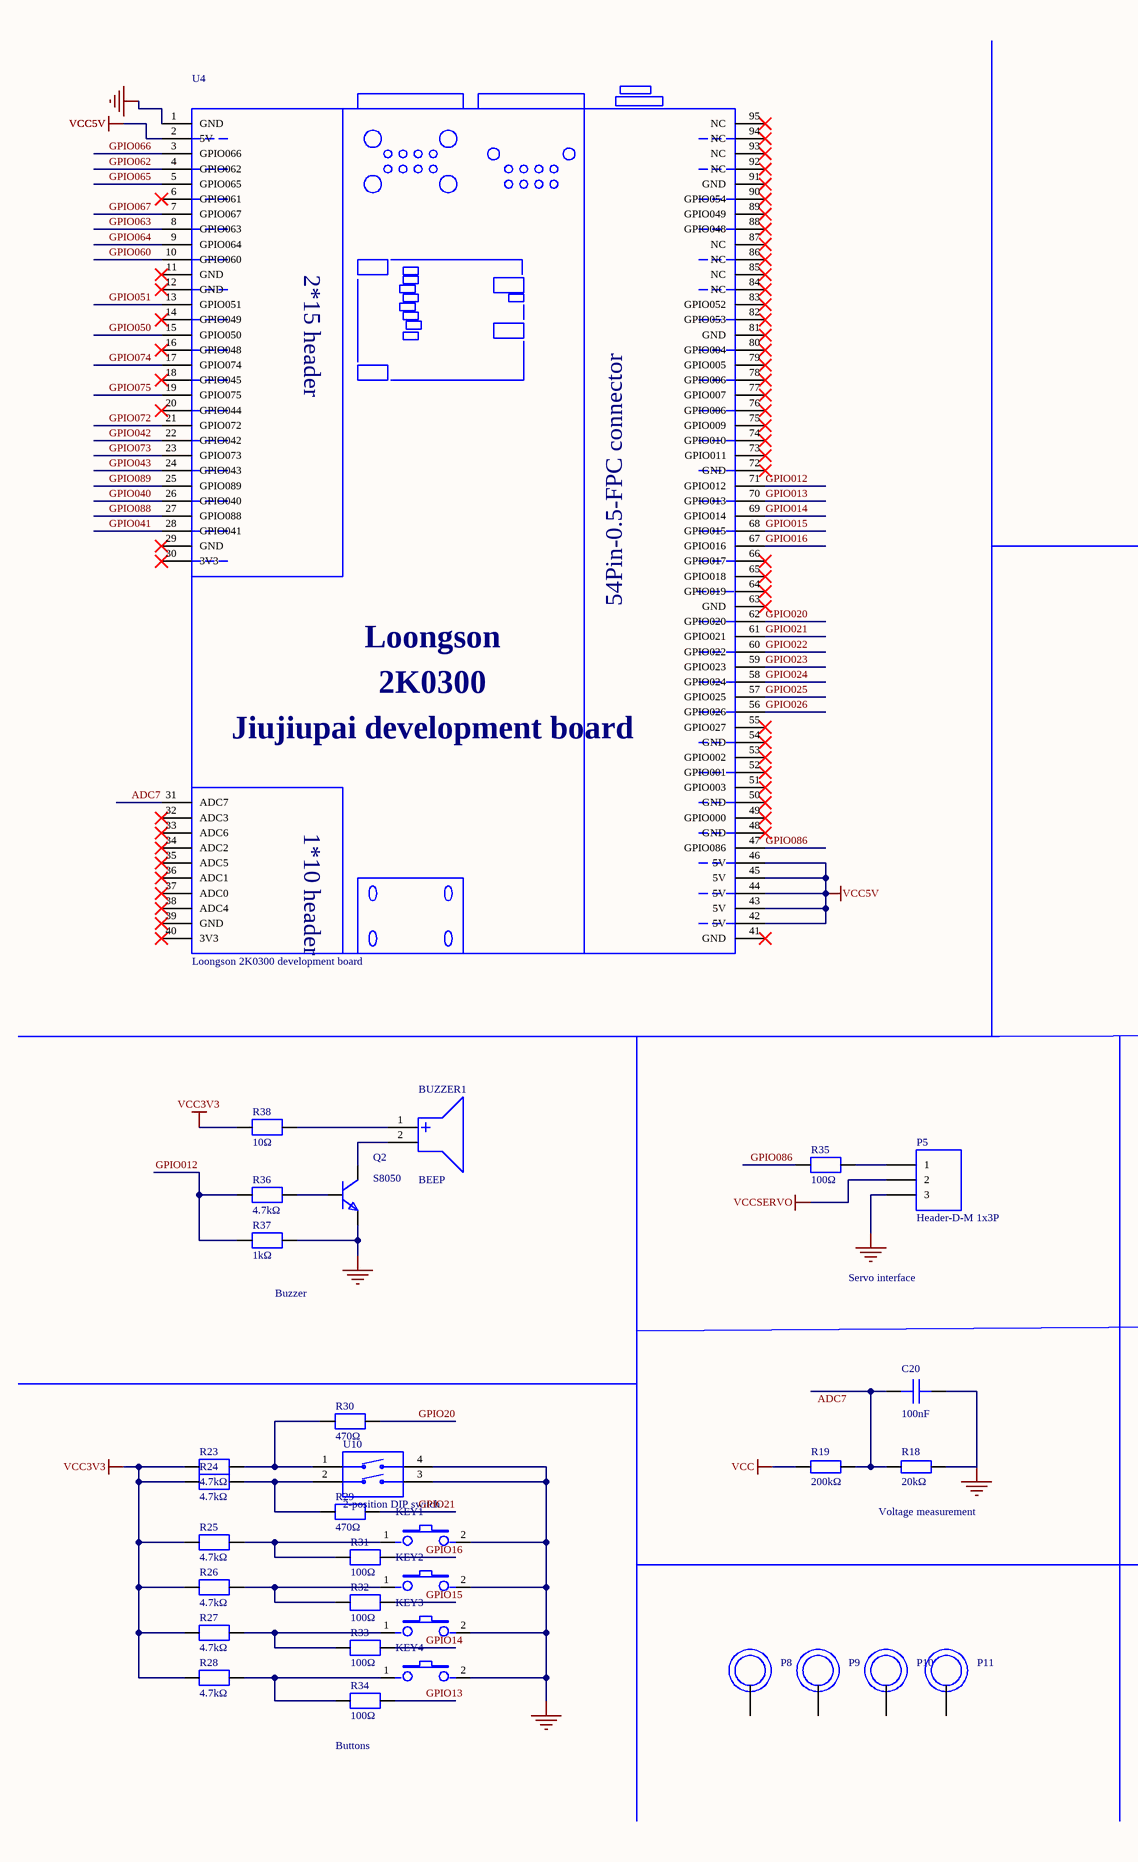
[diagram p0: MISC62349-3.schdoc, left]
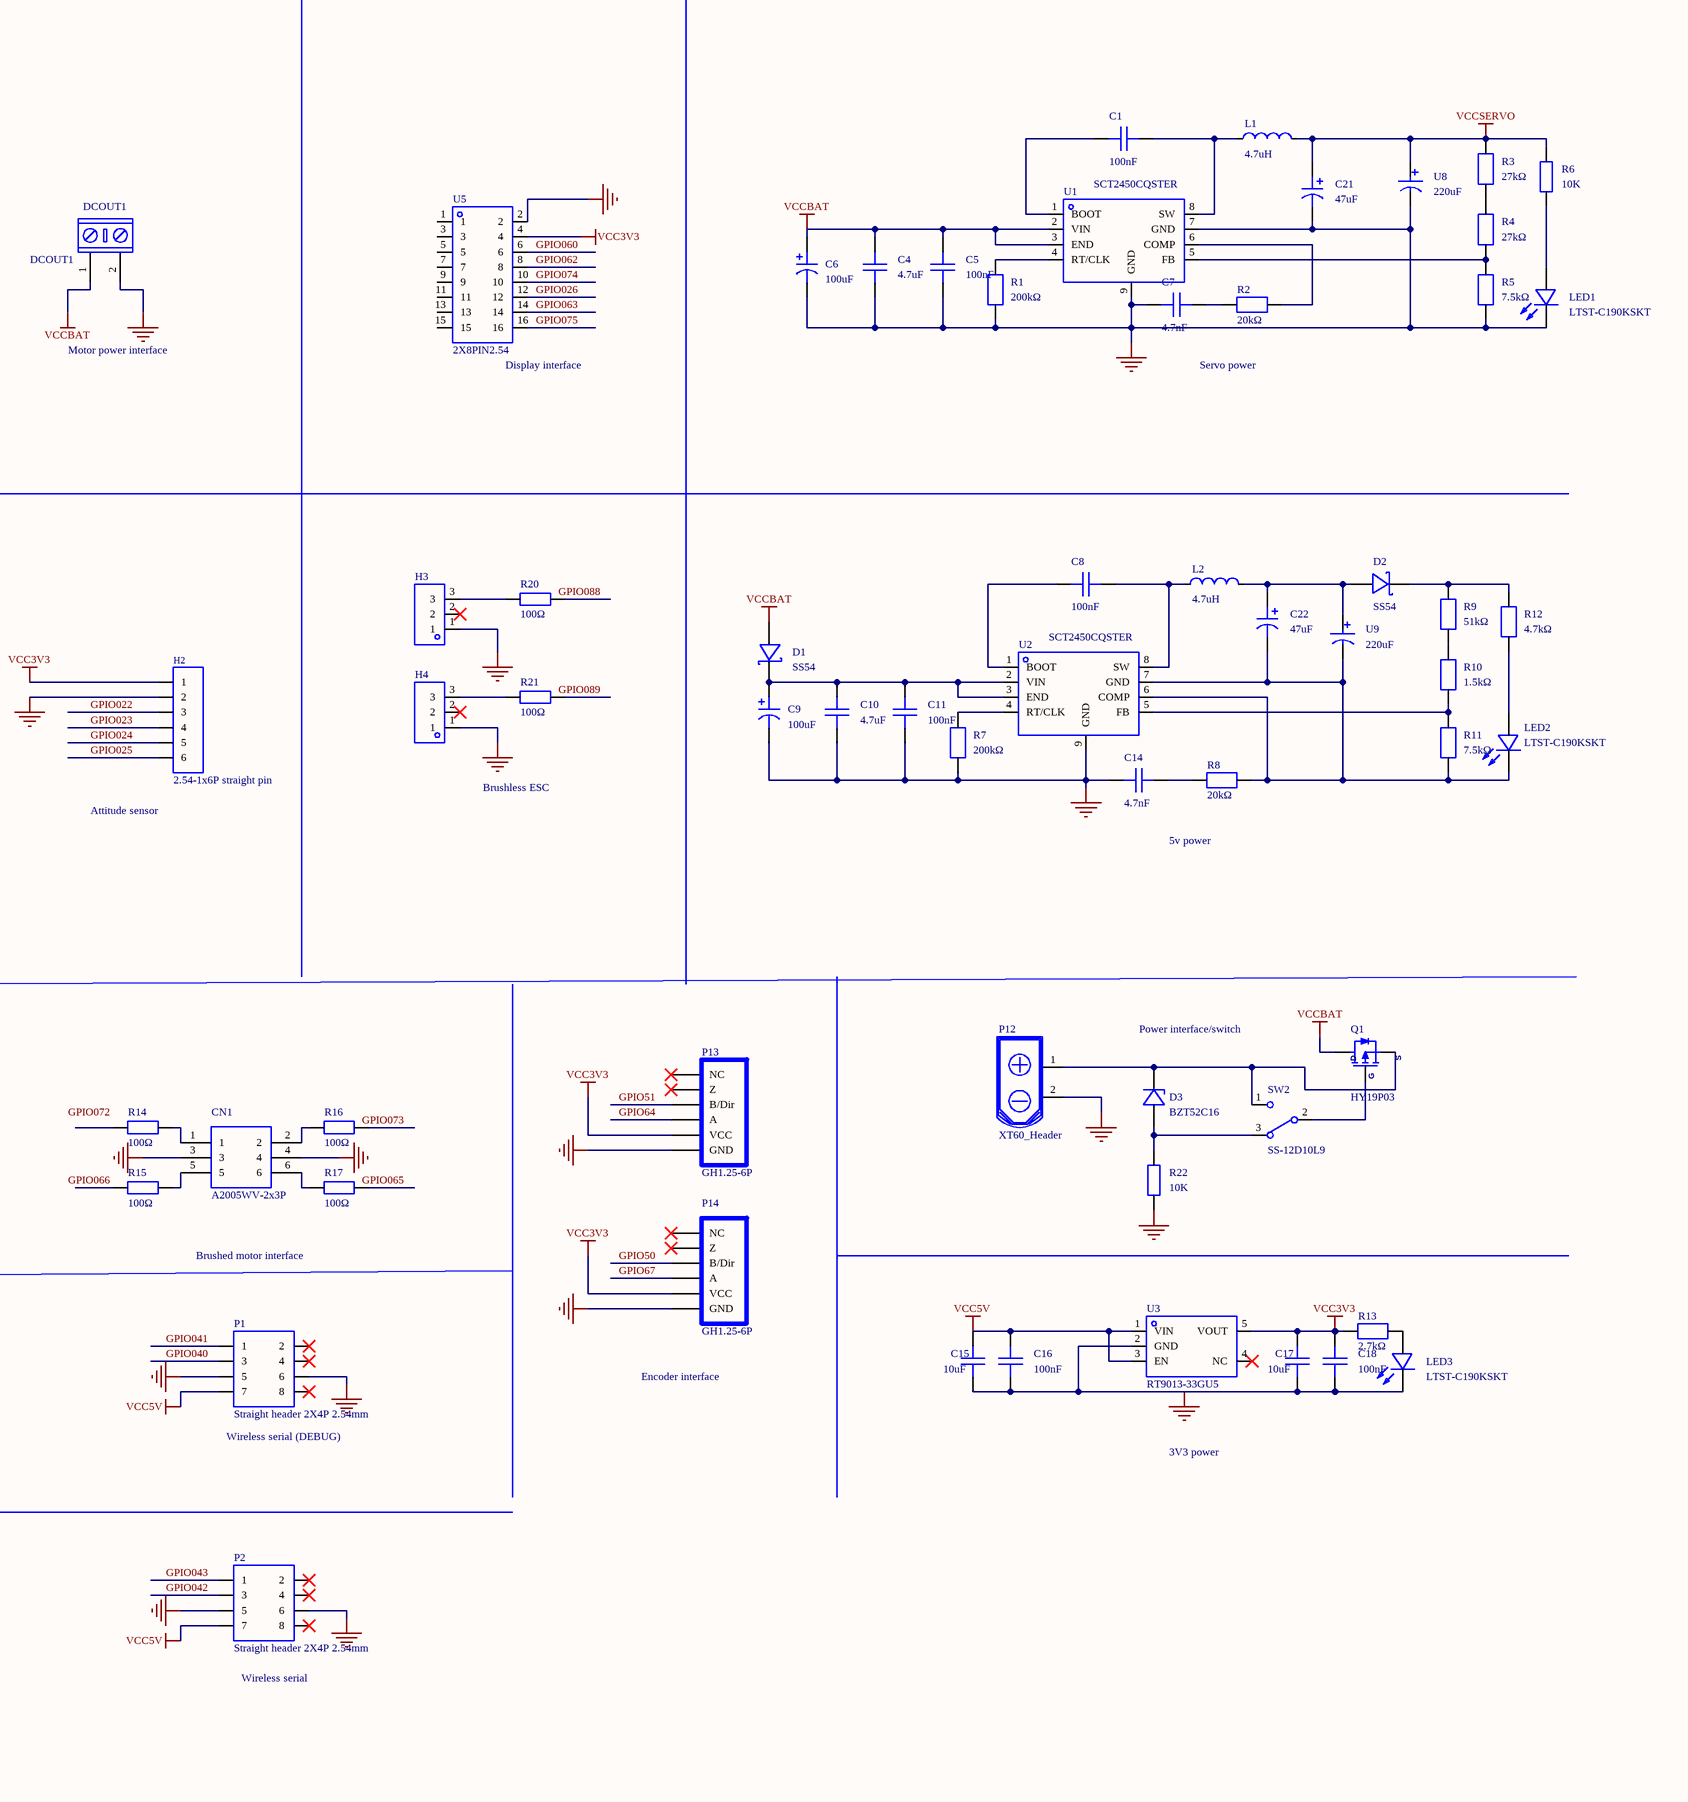
[diagram p1: MISC62349-3.schdoc, right]
# Altium project MISC62349-2.PrjPcb
1 sheet, 94 parts. Net scope: global (net labels, ports and power ports of the same name join across sheets).
Board file: MISC62349.pcbdoc

## Sheet MISC62349-3.schdoc
size 457 x 305 mm; Version: V1.0; @Project Name: MISC62349; @Page Count: 1; @Update Date: 2025-06-04; @Create Date: 2025-06-04; @Schematic Name: MISC62349; @Page No: 1; @Create Time: 18:07:27; @Update Time: 20:53:52; @Board Name: MISC62349

### Parts
BUZZER1  BEEP  [BUZ-TH_BD9-P50-D0.6-FD]
C1  100nF  [C0603]
C4  4.7uF  [C0402]
C5  100nF  [C0603]
C6  100uF  [CAP-SMD_L3.5-W2.8-R-RD]
C7  4.7nF  [C0603]
C8  100nF  [C0603]
C9  100uF  [CAP-SMD_L3.5-W2.8-R-RD]
C10  4.7uF  [C0402]
C11  100nF  [C0603]
C14  4.7nF  [C0603]
C15  10uF  [C0805]
C16  100nF  [C0603]
C17  10uF  [C0805]
C18  100nF  [C0603]
C20  100nF  [C0603]
C21  47uF  [CAP-SMD_BD6.3-L6.6-W6.6-LS7.3-FD]
C22  47uF  [CAP-SMD_BD6.3-L6.6-W6.6-LS7.3-FD]
CN1  A2005WV-2x3P  [HDR-TH_6P-P2.00-V-M-R2-C3-S2.00]
D1  SS54  [SMA_L4.4-W2.8-LS5.4-R-RD]
D2  SS54  [SMA_L4.4-W2.8-LS5.4-R-RD]
D3  BZT52C16  [SOD-123-L]
DCOUT1  DCOUT1  [KF/WJ/DG 301-2P-5.0MM]
H2  2.54-1x6P straight pin  [HDR-TH_6P-P2.54-V-M-1]
H3  (no value)  [HDR-TH_3P-P2.54-V-M]
H4  (no value)  [HDR-TH_3P-P2.54-V-M]
KEY1  Tact switch 3x6x2.5mm  [SW-SMD_L6.0-W3.6-LS8.0]  (value not drawn)
KEY2  Tact switch 3x6x2.5mm  [SW-SMD_L6.0-W3.6-LS8.0]  (value not drawn)
KEY3  Tact switch 3x6x2.5mm  [SW-SMD_L6.0-W3.6-LS8.0]  (value not drawn)
KEY4  Tact switch 3x6x2.5mm  [SW-SMD_L6.0-W3.6-LS8.0]  (value not drawn)
L1  4.7uH  [IND-SMD_L7.0-W6.6_VCMT063T]
L2  4.7uH  [IND-SMD_L7.0-W6.6_VCMT063T]
LED1  LTST-C190KSKT  [LED0603-RD]
LED2  LTST-C190KSKT  [LED0603-RD]
LED3  LTST-C190KSKT  [LED0603-RD]
P1  Straight header 2X4P 2.54mm  [HDR-TH_8P-P2.54-V-M-R2-C4-S2.54]
P2  Straight header 2X4P 2.54mm  [HDR-TH_8P-P2.54-V-M-R2-C4-S2.54]
P5  Header-D-M 1x3P  [HDR1X3-M]
P8  (no value)  [定位孔]
P9  (no value)  [定位孔]
P10  (no value)  [定位孔]
P11  (no value)  [定位孔]
P12  XT60_Header  [Wired T-Header ThroughHole]
P13  GH1.25-6P  [ECD-GH1.25-6P-SH]
P14  GH1.25-6P  [ECD-GH1.25-6P-SH]
Q1  HY19P03  [TO-252AA]
Q2  S8050  [SOT-23(SOT-23-3)]
R1  200kΩ  [R0603]
R2  20kΩ  [R0603]
R3  27kΩ  [R0603]
R4  27kΩ  [R0603]
R5  7.5kΩ  [R0603]
R6  10K  [R0603]
R7  200kΩ  [R0603]
R8  20kΩ  [R0603]
R9  51kΩ  [R0603]
R10  1.5kΩ  [R0603]
R11  7.5kΩ  [R0603]
R12  4.7kΩ  [R0603]
R13  2.7kΩ  [R0603]
R14  100Ω  [R0603]
R15  100Ω  [R0603]
R16  100Ω  [R0603]
R17  100Ω  [R0603]
R18  20kΩ  [R0603]
R19  200kΩ  [R0603]
R20  100Ω  [R0603]
R21  100Ω  [R0603]
R22  10K  [R0603]
R23  4.7kΩ  [R0603]
R24  4.7kΩ  [R0603]
R25  4.7kΩ  [R0603]
R26  4.7kΩ  [R0603]
R27  4.7kΩ  [R0603]
R28  4.7kΩ  [R0603]
R29  470Ω  [R0603]
R30  470Ω  [R0603]
R31  100Ω  [R0603]
R32  100Ω  [R0603]
R33  100Ω  [R0603]
R34  100Ω  [R0603]
R35  100Ω  [R0603]
R36  4.7kΩ  [R0603]
R37  1kΩ  [R0603]
R38  10Ω  [R0603]
SW2  SS-12D10L9  [MTS-10x]
U1  SCT2450CQSTER  [ESOP-8_L4.9-W3.9-P1.27-LS6.0-BL-EP]
U2  SCT2450CQSTER  [ESOP-8_L4.9-W3.9-P1.27-LS6.0-BL-EP]
U3  RT9013-33GU5  [SC-70-5_L2.0-W1.3-P0.65-LS2.1-BR]
U4  Loongson 2K0300 development board  [龙芯2K0300久久派开发板]
U5  2X8PIN2.54  [HDR-TH_16P-P2.54-V-M-R2-C8-S2.54]
U8  220uF  [CAP-SMD_BD6.3-L6.6-W6.6-LS7.2-FD]
U9  220uF  [CAP-SMD_BD6.3-L6.6-W6.6-LS7.2-FD]
U10  2-position DIP switch  [SW-TH_4P-L9.9-W6.8-P7.62-BL]

### Nets
GND: C4.1 C5.1 C6.2 C7.1 C9.2 C10.1 C11.1 C14.1 C15.1 C16.1 C17.1 C18.1 C20.2 C21.2 CN1.3 CN1.4 DCOUT1.2 H2.2 H3.1 H4.1 KEY1.2 KEY2.2 KEY3.2 KEY4.2 LED1.1(-) LED3.1(-) P1.5 P1.6 P2.5 P2.6 P5.3 P12.2(-) P13.1(GND) P14.1(GND) Q2.2(E) R1.1 R5.1 R7.1 R18.2 R22.1 R37.2 U1.7(GND) U1.9(GND) U2.9(GND) U3.2(GND) U4.1(GND) U5.2 U8.2 U10.3 U10.4
VCC: R19.1
VCC3V3: C17.2 C18.2 H2.1 P13.2(VCC) P14.2(VCC) R13.1 R23.1 R24.1 R25.1 R26.1 R27.1 R28.1 R38.1 U3.5(VOUT) U5.4
VCC5V: C15.2 C16.2 P1.7 P2.7 U3.1(VIN) U3.3(EN) U4.2(5V) U4.42(5V) U4.43(5V) U4.44(5V) U4.45(5V) U4.46(5V)
VCCBAT: C4.2 C5.2 C6.1 D1.1(A) DCOUT1.1 Q1.1(D) U1.2(VIN) U1.3(END)
VCCSERVO: C21.1 L1.2 P5.2 R3.2 R6.2 U8.1
ADC7: C20.1 R18.1 R19.2 U4.31(ADC7)
GPIO012: U4.71(GPIO012)
GPIO013: U4.70(GPIO013)
GPIO13: R34.2
GPIO014: U4.69(GPIO014)
GPIO14: R33.2
GPIO015: U4.68(GPIO015)
GPIO15: R32.2
GPIO016: U4.67(GPIO016)
GPIO16: R31.2
GPIO020: U4.62(GPIO020)
GPIO20: R30.2
GPIO021: U4.61(GPIO021)
GPIO21: R29.2
GPIO022: H2.3 U4.60(GPIO022)
GPIO023: H2.4 U4.59(GPIO023)
GPIO024: H2.5 U4.58(GPIO024)
GPIO025: H2.6 U4.57(GPIO025)
GPIO026: U4.56(GPIO026) U5.12
GPIO040: P1.3 U4.26(GPIO040)
GPIO041: P1.1 U4.28(GPIO041)
GPIO042: P2.3 U4.22(GPIO042)
GPIO043: P2.1 U4.24(GPIO043)
GPIO050: U4.15(GPIO050)
GPIO50: P14.4(B/Dir)
GPIO051: U4.13(GPIO051)
GPIO51: P13.4(B/Dir)
GPIO060: U4.10(GPIO060) U5.6
GPIO062: U4.4(GPIO062) U5.8
GPIO063: U4.8(GPIO063) U5.14
GPIO064: U4.9(GPIO064)
GPIO64: P13.3(A)
GPIO065: U4.5(GPIO065)
GPIO066: U4.3(GPIO066)
GPIO067: U4.7(GPIO067)
GPIO67: P14.3(A)
GPIO072: U4.21(GPIO072)
GPIO073: U4.23(GPIO073)
GPIO074: U4.17(GPIO074) U5.10
GPIO075: U4.19(GPIO075) U5.16
GPIO086: R35.1 U4.47(GPIO086)
GPIO088: U4.27(GPIO088)
GPIO089: U4.25(GPIO089)
NetBUZZER1_1: BUZZER1.1(+) R38.2
NetBUZZER1_2: BUZZER1.2(-) Q2.3(C)
NetC1_1: C1.1 U1.1(BOOT)
NetC1_2: C1.2 L1.1 U1.8(SW)
NetC7_2: C7.2 R2.2
NetC8_1: C8.1 U2.1(BOOT)
NetC8_2: C8.2 L2.1 U2.8(SW)
NetC9_1: C9.1 C10.2 C11.2 D1.2(K) U2.2(VIN) U2.3(END)
NetC14_2: C14.2 R8.2
NetC22_1: C22.1 D2.1(A) L2.2 U9.1
NetC22_2: C22.2 LED2.1(-) R8.1 R11.1 U2.6(COMP) U2.7(GND) U9.2
NetCN1_1: CN1.1 R14.2
NetCN1_2: CN1.2 R16.1
NetCN1_5: CN1.5 R15.2
NetCN1_6: CN1.6 R17.1
NetD2_2: D2.2(K) R9.2 R12.2
NetD3_A: D3.A R22.2 SW2.3
NetD3_K: D3.K P12.1(+) Q1.3(S) SW2.1
NetH3_3: H3.3 R20.1
NetH4_3: H4.3 R21.1
NetKEY1_1: KEY1.1 R25.2 R31.1
NetKEY2_1: KEY2.1 R26.2 R32.1
NetKEY3_1: KEY3.1 R27.2 R33.1
NetKEY4_1: KEY4.1 R28.2 R34.1
NetLED1_2: LED1.2(+) R6.1
NetLED2_2: LED2.2(+) R12.1
NetLED3_2: LED3.2(+) R13.2
NetP5_1: P5.1 R35.2
NetQ1_2: Q1.2(G) SW2.2
NetQ2_1: Q2.1(B) R36.2
NetR1_2: R1.2 U1.4(RT/CLK)
NetR2_1: R2.1 U1.6(COMP)
NetR3_1: R3.1 R4.2
NetR4_1: R4.1 R5.2 U1.5(FB)
NetR7_2: R7.2 U2.4(RT/CLK)
NetR9_1: R9.1 R10.2
NetR10_1: R10.1 R11.2 U2.5(FB)
NetR23_2: R23.2 R30.1 U10.1
NetR24_2: R24.2 R29.1 U10.2
NetR36_1: R36.1 R37.1

Not connected (* = marked no-connect by the designer): H3 2*; H4 2*; P1 2* 4* 8*; P2 2* 4* 8*; P8 1; P9 1; P10 1; P11 1; P13 5(Z)* 6(NC)*; P14 5(Z)* 6(NC)*; R14 1; R15 1; R16 2; R17 2; R20 2; R21 2; U3 4(NC)*; U4 6(GPIO061)* 11(GND)* 12(GND)* 14(GPIO049)* 16(GPIO048)* 18(GPIO045)* 20(GPIO044)* 29(GND)* 30(3V3)* 32(ADC3)* 33(ADC6)* 34(ADC2)* 35(ADC5)* 36(ADC1)* 37(ADC0)* 38(ADC4)* 39(GND)* 40(3V3)* 41(GND)* 48(GND)* 49(GPIO000)* 50(GND)* 51(GPIO003)* 52(GPIO001)* 53(GPIO002)* 54(GND)* 55(GPIO027)* 63(GND)* 64(GPIO019)* 65(GPIO018)* 66(GPIO017)* 72(GND)* 73(GPIO011)* 74(GPIO010)* 75(GPIO009)* 76(GPIO006)* 77(GPIO007)* 78(GPIO006)* 79(GPIO005)* 80(GPIO004)* 81(GND)* 82(GPIO053)* 83(GPIO052)* 84(NC)* 85(NC)* 86(NC)* 87(NC)* 88(GPIO048)* 89(GPIO049)* 90(GPIO054)* 91(GND)* 92(NC)* 93(NC)* 94(NC)* 95(NC)*; U5 1 3 5 7 9 11 13 15

### Notes on the sheet
- Motor power interface
- (near U5) Display interface
- Servo power
- (near H2) Attitude sensor
- Brushless ESC
- 5v power
- Power interface/switch
- (near R37) Buzzer
- Servo interface
- Brushed motor interface
- (near P1) Wireless serial (DEBUG)
- Encoder interface
- Voltage measurement
- 3V3 power
- (near R34) Buttons
- (near P2) Wireless serial
- Labels drawn without touching a wire or pin: GPIO012, GPIO065, GPIO066, GPIO072, GPIO073, GPIO088, GPIO089
- 2025-06-04
- Schematic
- Board
- Sheet
- P1
- Drawn
- Reviewed
- Revision
- Size
- A4
- page 1 Total 1
- EDA

### Library data of the parts
BUZZER1 = BEEP: ManufacturerPart: 5V,管脚间距8mm,外径10mm,高9.5mm; AddInBom: yes; ModelId: 638ddae033e2460c89b09f6fe40a11c2; ModelName: BUZ-TH_BD9.0-P5.00-D0.6-L-FD; ModelTransform: 354.33,354.13,433.07,90,0,0,0,0,-212.6; Device: BEEP; LCSC Part Name: 5V,管脚间距8mm,外径10mm,高9.5mm; SupplierPart: C9900017013; Supplier Footprint: BEEP; Supplier: LCSC; ConvertToPcb: yes; SymbolName: BEEP; FootprintName: BUZ-TH_BD9-P50-D0.6-FD
C1 C5 C8 C11 C16 C18 = 06031C104K4T2A: Capacitance:100nF;Tolerance:±10%;Rated voltage:100V;Temp coefficient:X7R;; Manufacturer: Kyocera AVX; AddInBom: yes; ModelId: ac125912035d415993ca9572d50418b1; ModelName: C0603_L1.6-W0.8-H0.8; ModelTransform: 62.992,31.496,0,0,0,0,0,0,0; Tolerance: ±10%; Voltage Rating: 100V; Temperature Coefficient: X7R; Symbol: 06031C104K4T2A; Device: 06031C104K4T2A; LCSC Part Name: 100nF ±10% 100V; SupplierPart: C1880996; ManufacturerPart: 06031C104K4T2A; Supplier Footprint: 0603; JLCPCB Part Class: Extended library; Supplier: LCSC; ConvertToPcb: yes; FootprintName: C0603; Value: 100nF
C4 C10 = 0402X475M160NT: Capacitance:4.7uF;Tolerance:±20%;Rated voltage:16V;Temp coefficient:X5R;; Manufacturer: FH(风华); AddInBom: yes; ModelId: 36a51122f27c49738f86b3bfa98863e0; ModelName: C0402_L1.0-W0.5-H0.5; ModelTransform: 39.37,19.685,0,0,0,0,0,0,0; Tolerance: ±20%; Voltage Rating: 16V; Temperature Coefficient: X5R; Symbol: 0402X475M160NT; Device: 0402X475M160NT; LCSC Part Name: 4.7uF ±20% 16V; SupplierPart: C2936654; ManufacturerPart: 0402X475M160NT; Supplier Footprint: 0402; JLCPCB Part Class: Extended library; Datasheet: https://atta.szlcsc.com/upload/public/pdf/source/20211229/0F554F04CCCC73F7B111AB47B2AF3160.pdf; Supplier: LCSC; ConvertToPcb: yes; FootprintName: C0402; Value: 4.7uF
C6 C9 = 8TPE100MAZB: Capacitance:100uF;Tolerance:±20%;Rated voltage:8V;Equivalent series resistance (ESR):35mΩ@100kHz;; Manufacturer: PANASONIC(松下); AddInBom: yes; ModelId: 0dfcda272f9b43668c6086d3a08712ba; ModelName: CASE-B_L3.5-W2.8-H1.9; ModelTransform: 145.669,110.236,0,180,0,0,0,0,0; Tolerance: ±20%; Voltage Rating: 8V; Symbol: 8TPE100MAZB; Device: 8TPE100MAZB; LCSC Part Name: 100uF ±20% 8V MSL=3拆包后请尽快使用; SupplierPart: C2158532; ManufacturerPart: 8TPE100MAZB; Supplier Footprint: 1411; JLCPCB Part Class: Extended library; Datasheet: https://atta.szlcsc.com/upload/public/pdf/source/20180730/C242097_33E927DF965764BEE6DB6E1D200BB8FE.pdf; Supplier: LCSC; ConvertToPcb: yes; FootprintName: CAP-SMD_L3.5-W2.8-R-RD; Value: 100uF; Current - Leakage: -; Ripple Current: -; Equivalent Series Resistance(ESR): 35mΩ@100kHz; Operating Temperature: -55℃~+105℃
C7 C14 = 0603CG472J500NT: Capacitance:4.7nF;Tolerance:±5%;Rated voltage:50V;Temp coefficient:C0G;; Manufacturer: FH(风华); AddInBom: yes; ModelId: ac125912035d415993ca9572d50418b1; ModelName: C0603_L1.6-W0.8-H0.8; ModelTransform: 62.992,31.496,0,0,0,0,0,0,0; Tolerance: ±5%; Voltage Rating: 50V; Temperature Coefficient: C0G; Symbol: 0603CG472J500NT; Device: 0603CG472J500NT; LCSC Part Name: 4.7nF ±5% 50V; SupplierPart: C20624280; ManufacturerPart: 0603CG472J500NT; Supplier Footprint: 0603; JLCPCB Part Class: Extended library; Datasheet: https://atta.szlcsc.com/upload/public/pdf/source/20231013/50987BFA113EBC42343E989A0A057269.pdf; Supplier: LCSC; ConvertToPcb: yes; FootprintName: C0603; Value: 4.7nF
C15 C17 = C0805X106K8RACAUTO: Capacitance:10uF;Tolerance:±10%;Rated voltage:10V;Temp coefficient:X7R;; Manufacturer: KEMET(基美); AddInBom: yes; ModelId: 1ba041120af144c991958decab20d241; ModelName: C0805_L2.0-W1.3-H1.3; ModelTransform: 78.74,51.181,0,0,0,0,0,0.0005,0; Tolerance: ±10%; Voltage Rating: 10V; Temperature Coefficient: X7R; Symbol: C0805X106K8RACAUTO; Device: C0805X106K8RACAUTO; LCSC Part Name: 10uF ±10% 10V; SupplierPart: C2167871; ManufacturerPart: C0805X106K8RACAUTO; Supplier Footprint: 0805; JLCPCB Part Class: Extended library; Datasheet: https://atta.szlcsc.com/upload/public/pdf/source/20210401/7F57E742531715B36FE1E9CC2258952B.pdf; Supplier: LCSC; ConvertToPcb: yes; FootprintName: C0805; Value: 10uF
C20 = CAP_0603: ConvertToPcb: yes; SymbolName: CapAcitance; ModelId: ac125912035d415993ca9572d50418b1; ModelName: C0603_L1.6-W0.8-H0.8; ModelTransform: 62.992,31.496,0,0,0,0,0,0,0; Device: CAP_0603; AddInBom: yes; Supplier Footprint: 0603; FootprintName: C0603; Value: 100nF
C21 C22 = SPT1CM470E05TRVZC: Capacitance:47uF;Tolerance:±20%;Rated voltage:16V;Type:Polymer;; Manufacturer: Yunxing(云星); AddInBom: yes; ModelId: 697a8c63e3274188b68c96045bc3ea1c; ModelTransform: 287.401,259.842,0,180,0,0,0.001,0.001,0; Tolerance: ±20%; Voltage Rated: 16V; Lifetime @ Temp: 2000hrs@105℃; Symbol: SPT1CM470E05TRVZC; Device: SPT1CM470E05TRVZC; LCSC Part Name: 47uF ±20% 16V; SupplierPart: C41410186; ManufacturerPart: SPT1CM470E05TRVZC; Supplier Footprint: SMD,D6.3xL5mm; Datasheet: https://atta.szlcsc.com/upload/public/pdf/source/20240919/E10B786B053F2EF740092A8DAB1988C9.pdf; Supplier: LCSC; ConvertToPcb: yes; FootprintName: CAP-SMD_BD6.3-L6.6-W6.6-LS7.3-FD; ModelName: CAP-SMD_BD6.3-L6.6-W6.6-LS7.3-FD; Value: 47uF; Type: Polymer; Diameter: 6.3mm; Height - Seated (Max): 5mm; Operating Temperature: -55℃~+105℃
CN1 = A2005WV-2x3P: 间距:2mm;总PIN位数:6;排数:2;插针结构:2x3P;行距:2mm;安装类型:直插;圆针/方针:方针;额定电流:-;额定电压:-;配合针长度:4mm;塑高:-;端接针长度:2.8mm;触头材质:黄铜;触头镀层:金;工作温度范围:-40℃~+105℃;颜色:黑色;; Manufacturer: CJT(长江连接器); AddInBom: yes; ModelId: 7bb0589f04a2434cbd3f756f04868c86; ModelName: HDR-TH_6P-P2.00-M-LI-2X3P; ModelTransform: 236.22,157.48,0,0,0,0,0,0,-118.11; Pitch: 2mm; Pin Structure: 2x3P; Circluar Pins/Square Pins: Square pin; Device: A2005WV-2x3P; Symbol: A2005WV-2X3P; LCSC Part Name: 2mm 2x3P 直插 方针 镀金; SupplierPart: C225288; ManufacturerPart: A2005WV-2x3P; Supplier Footprint: 插件,P=2mm; JLCPCB Part Class: Extended Part; Datasheet: https://atta.szlcsc.com/upload/public/pdf/source/20180509/C225288_5A34F913C29FC1A6DA0E0F7E9D3856BA.pdf; Supplier: LCSC; ConvertToPcb: yes; FootprintName: HDR-TH_6P-P2.00-V-M-R2-C3-S2.00; Number of Pins: 6; Number of Rows: 2; Row Spacing: 2mm; Mounting Type: Through-hole; Current Rating (Max): -; Voltage Rating (Max): -; Length of Mating Pin: 4mm; Insulation Height: -; Length of End Connection Pin: 2.8mm; Contact Material: Brass; Contact Plating: Gold; Operating Temperature Range: -40℃~+105℃; Color: Black
D1 D2 = SS54_C22452: Diode configuration:Single;Forward voltage drop (Vf):550mV@5A;DC reverse voltage (Vr):40V;Rectified current:5A;; Manufacturer: MDD(辰达半导体); AddInBom: yes; ModelId: 228de99b63224bd3982b21290755dd84; ModelTransform: 204.724,110.236,0,0,0,0,0,0,0; Diode Configuration: Single; Reverse Voltage (Vr): 40V; Rectified Current: 5A; Reverse Leakage Current (Ir): 1mA@40V; Symbol: SS54_C22452; Device: SS54_C22452; LCSC Part Name: 电压:40V 电流:5A; SupplierPart: C22452; ManufacturerPart: SS54; Supplier Footprint: SMA(DO-214AC); JLCPCB Part Class: Basic library; Datasheet: https://atta.szlcsc.com/upload/public/pdf/source/20240710/73DFBB65C1883B895E62D589679033DF.pdf; Supplier: LCSC; ConvertToPcb: yes; FootprintName: SMA_L4.4-W2.8-LS5.4-R-RD; ModelName: SMA_L4.4-W2.8-LS5.4-R-RD; Forward Voltage (Vf@If): 550mV@5A
D3 = BZT52C16: Origin Footprint 2: DIODE-0.7; Origin Footprint 3: DIODE-0.4; Origin Footprint 4: SOD-87[LL-41]; Origin Footprint 5: CD4521-1808; Origin Footprint 6: SOD-80[LL-34]; Origin Footprint 7: SOD-123-FL; Origin Footprint 8: SOD-123-M; Origin Footprint 9: SOD-323; Origin Footprint 10: SOD-523-L; Origin Footprint 11: SOD-523-M; AddInBom: yes; SymbolName: Diode Zen; Device: BZT52C16; Published: 8-Jun-2000; Revision: July-2002: Re-released for DXP Platform.; Price(RMB): 0.000; ConvertToPcb: yes; FootprintName: SOD-123-L; Publisher: Altium Limited
DCOUT1 = DCOUT1: AddInBom: yes; Device: DCOUT1; ConvertToPcb: yes; SymbolName: DCOUT1; FootprintName: KF/WJ/DG 301-2P-5.0MM
H2 = 2.54-1x6P直针: 间距:2.54mm;总PIN位数:6;排数:1;插针结构:1x6P;行距:-;安装类型:直插;圆针/方针:方针;额定电流:3A;额定电压:-;配合针长度:-;塑高:-;触头材质:黄铜;触头镀层:-;工作温度范围:-40℃~+105℃;颜色:黑色;; Manufacturer: BOOMELE(博穆精密); Symbol: Header-Male-2.54_1x6; AddInBom: yes; ModelId: 60739dffc9b04830a286435b0fefbd4a; ModelName: HDR2.54-M-LI-1X6P; ModelTransform: 600,100,0,0,0,0,0,0,-118.1; Pitch: 2.54mm; Pin Structure: 1x6P; Circluar Pins/Square Pins: Square pin; Current Rating (Max): 3A; Device: 2.54-1x6P straight pin; Supplier: LCSC; Manufacturer Part: 2.54-1x6P直针; Supplier Part: C37208; JLCPCB Part Class: Extended Part; LCSC Part Name: 2.54mm 1x6P 直插 方针; Supplier Footprint: 直插,P=2.54mm; Datasheet: https://atta.szlcsc.com/upload/public/pdf/source/20151109/1457707558014.pdf; ConvertToPcb: yes; FootprintName: HDR-TH_6P-P2.54-V-M-1; Number of Pins: 6; Number of Rows: 1; Row Spacing: -; Mounting Type: Through-hole; Voltage Rating (Max): -; Length of Mating Pin: -; Insulation Height: -; Contact Material: Brass; Contact Plating: -; Operating Temperature Range: -40℃~+105℃; Color: Black
H3 H4 = HDR-M_2.54_1x3P: Symbol: PZ254V-11-03P_C2937625; ConvertToPcb: yes; ModelId: bb473b6d38ff42a99216a4fcdbdcc4cb; ModelName: HDR-TH_3P-P2.54-M-LI-1X3P; ModelTransform: 299.9994,100,0,0,0,0,0,0,-118.11; Device: HDR-M_2.54_1x3P; AddInBom: yes; SupplierPart: C2937625; Supplier Footprint: 插件; FootprintName: HDR-TH_3P-P2.54-V-M
KEY1-KEY4 = 轻触按键 3x6x2.5mm: AddInBom: yes; ModelId: 5cda64a5897044e48badc24f5aa7d420; ModelName: SW-SMD_L6.0-W3.6-H2.5-LS8.0; ModelTransform: 314.96,141.732,0,0,0,0,0,0,0; Symbol: 3x6x2.5mm; Device: Tact switch 3x6x2.5mm; LCSC Part Name: 3x6x2.5 红头 耐高温; SupplierPart: C5382; ManufacturerPart: 轻触按键 3x6x2.5mm; Supplier Footprint: SMD; JLCPCB Part Class: Extended library; Supplier: LCSC; ConvertToPcb: yes; FootprintName: SW-SMD_L6.0-W3.6-LS8.0
L1 L2 = ZEMS0603-4R7M: Inductance:4.7uH;Tolerance:±20%;Rated current:6A;Saturation current (Isat):9A;Type:Molded inductor;; Manufacturer: ZE(增益); AddInBom: yes; ModelId: f4285975b224408e9720a50707b42a76; ModelTransform: 275.59,260.2357,0,0,0,0,0,0,0; Tolerance: ±20%; Current Rating: 6A; Current - Saturation(Isat): 9A; DC Resistance(DCR): 40mΩ; Symbol: ZEMS0603-4R7M; Device: ZEMS0603-4R7M; LCSC Part Name: ZEMS0603-4R7M; SupplierPart: C41415578; ManufacturerPart: ZEMS0603-4R7M; Supplier Footprint: SMD,7x6.6mm; Datasheet: https://atta.szlcsc.com/upload/public/pdf/source/20241008/E174FBE73995C1DD66BAC4D7D2F842CD.pdf; Supplier: LCSC; ConvertToPcb: yes; FootprintName: IND-SMD_L7.0-W6.6_VCMT063T; ModelName: IND-SMD_L7.0-W6.6_VCMT063T; Value: 4.7uH; Type: Molded inductor
LED1-LED3 = LTST-C190KSKT: 发光颜色:黄色;正向电压(VF):2.1V;功率:75mW;正向电流:20mA;主波长:584.5nm~597nm;二极管配置:-;透镜颜色:无色透明透镜;色温:-;发光强度:104mcd;发光角度:130°;载带方式:-;工作温度:-30℃~+85℃;; Manufacturer: LITEON(光宝); AddInBom: yes; ModelId: 1f0d29a91be547639d425604e9b96ebb; ModelTransform: 63.7794,32.283,0,0,0,0,0,0,0; Emitted Color: Yellow; Forward Voltage (VF): 2.1V; Power Dissipation: 75mW; Forward Current: 20mA; Peak Wavelength: 588nm; Lens Color: Clear lens; Luminous Intensity: 104mcd; Viewing Angle: 130°; Symbol: LTST-C190KSKT; Device: LTST-C190KSKT; LCSC Part Name: 黄灯; SupplierPart: C125095; ManufacturerPart: LTST-C190KSKT; Supplier Footprint: 0603; JLCPCB Part Class: Extended library; Datasheet: https://atta.szlcsc.com/upload/public/pdf/source/20180129/C125095_15171881843821315881.pdf; Supplier: LCSC; ConvertToPcb: yes; FootprintName: LED0603-RD; ModelName: LED0603-RD; Dominant Wavelength: 584.5nm~597nm; Diode Configuration: -; Color Temperature: -; Mounting Sytle: -; Operating Temperature: -30℃~+85℃
P1 P2 = 直排针2X4P 2.54mm: Rows:-;Round/square pin:-;Rated current:-;Rated voltage:-;Mating pin length:-;Plastic height:-;Contact material:-;; Manufacturer: BOOMELE(博穆精密); Symbol: Header-Male-2.54_2x4; AddInBom: yes; ModelId: 9655140a9899454ea9d6a6732d55fb0e; ModelName: HDR-TH_8P-P2.54-M-LI-2X4P; ModelTransform: 400,200,0,0,0,0,0,0,-118.1; Device: Straight header 2X4P 2.54mm; LCSC Part Name: 排针 2*4P 2.54mm; SupplierPart: C58363; ManufacturerPart: 直排针2X4P 2.54mm; Supplier Footprint: 插件,P=2.54mm; JLCPCB Part Class: Extended Part; Datasheet: https://atta.szlcsc.com/upload/public/pdf/source/20151026/1457707506726.pdf; Supplier: LCSC; ConvertToPcb: yes; FootprintName: HDR-TH_8P-P2.54-V-M-R2-C4-S2.54; Number of Rows: -; Circluar Pins/Square Pins: -; Current Rating (Max): -; Voltage Rating (Max): -; Length of Mating Pin: -; Insulation Height: -; Contact Material: -
P5 = Header-D-M 1x3P: 1x3pin, through-hole, pin header; AddInBom: yes; Device: Header-D-M 1x3P; Revision: V1.0; Value: Header-D-M 1x3P; Footprint Name: HDR1X3-M; ConvertToPcb: yes; SymbolName: Header-D-M 1x3P; FootprintName: HDR1X3-M
P8-P11 = 定位孔: Device: Locating hole; AddInBom: yes; ModelId: c0272a1083aa488a8080554edf29f67b; ModelName: SMD_SMTSO3060CTJ; ModelTransform: 218.897,218.387,0,0,0,0,-0.155,-0.01,-59.055; _: 3; ConvertToPcb: yes; SymbolName: Locating hole; FootprintName: Locating hole
P12 = XT60_Header: AddInBom: yes; Device: XT60_Header; Footprint Name: XT60UF; ConvertToPcb: yes; SymbolName: XT60_Header; FootprintName: Wired T-Header ThroughHole; Description: XT60_Header
P13 P14 = GH1.25-6P: COMPANY_A 1024-line encoder GH1.25-6P, board side; AddInBom: yes; SymbolName: GH1.25-6P-new encoder board side; Device: GH1.25-6P; Revision: V1.0; Value: GH1.25-6P; Footprint Name: ECD-GH1.25-6P-SV; ConvertToPcb: yes; FootprintName: ECD-GH1.25-6P-SH
Q1 = HY19P03: AddInBom: yes; Device: HY19P03; ConvertToPcb: yes; SymbolName: HY19P03; FootprintName: TO-252AA
Q2 = S8050: Manufacturer: CJ; AddInBom: yes; Device: S8050; ConvertToPcb: yes; SymbolName: S8050; Supplier: LCSC; ManufacturerPart: S8050; image: C2146.jpg; SupplierPart: C2146; JLCPCB Part Class: Basic; FootprintName: SOT-23(SOT-23-3)
R1 R7 = AF0805FR-07200KL: Resistor type:Thick film resistor;Resistance:200kΩ;Tolerance:±1%;Power:125mW;Temp coefficient:±100ppm/℃;; Manufacturer: YAGEO(国巨); AddInBom: yes; ModelId: 37a81e68749a4138bd2dfa6897b24b85; ModelName: R0805_L2.0-W1.3-H0.6; ModelTransform: 78.74,51.181,0,0,0,0,0,-0.0005,0; Tolerance: ±1%; Power(Watts): 125mW; Symbol: AF0805FR-07200KL; Device: AF0805FR-07200KL; LCSC Part Name: 厚膜电阻 200kΩ ±1% 125mW; SupplierPart: C3957483; ManufacturerPart: AF0805FR-07200KL; Supplier Footprint: 0805; JLCPCB Part Class: Extended library; Datasheet: https://atta.szlcsc.com/upload/public/pdf/source/20240124/9D5CBAA83CB4685F032349418AF2E20F.pdf; Supplier: LCSC; ConvertToPcb: yes; FootprintName: R0603; Type: Thick film resistor; Value: 200kΩ; Temperature Coefficient: ±100ppm/℃; Operating Temperature: -55℃~+155℃
R2 R8 = MMA02040D2002FB300: Resistor type:Thin film resistor;Resistance:20kΩ;Tolerance:±1%;Power:400mW;Working voltage:200V;Temp coefficient:±25ppm/℃;; Manufacturer: VISHAY(威世); AddInBom: yes; ModelId: bdd6039e5cb54d129162151e55f23c33; ModelName: R0204; ModelTransform: 137.795,55.09383,0,0,0,0,0,0,0; Tolerance: ±1%; Power(Watts): 400mW; Voltage-Supply(Max): 200V; Symbol: MMA02040D2002FB300; Device: MMA02040D2002FB300; LCSC Part Name: 薄膜电阻 20kΩ ±1% 400mW; SupplierPart: C2139897; ManufacturerPart: MMA02040D2002FB300; Supplier Footprint: 0204; JLCPCB Part Class: Extended library; Datasheet: https://atta.szlcsc.com/upload/public/pdf/source/20210505/324368DA0CE91162B72B5E4004EB06CA.pdf; Supplier: LCSC; ConvertToPcb: yes; FootprintName: R0603; Type: Thin film resistor; Value: 20kΩ; Temperature Coefficient: ±25ppm/℃; Operating Temperature: -55℃~+155℃
R3 R4 = RT0805BRE0727KL: Resistor type:Thin film resistor;Resistance:27kΩ;Tolerance:±0.1%;Power:125mW;Temp coefficient:±50ppm/℃;; Manufacturer: YAGEO(国巨); AddInBom: yes; ModelId: 37a81e68749a4138bd2dfa6897b24b85; ModelName: R0805_L2.0-W1.3-H0.6; ModelTransform: 78.74,51.181,0,0,0,0,0,-0.0005,0; Tolerance: ±0.1%; Power(Watts): 125mW; Symbol: RT0805BRE0727KL; Device: RT0805BRE0727KL; LCSC Part Name: 薄膜电阻 27kΩ ±0.1% 125mW; SupplierPart: C706273; ManufacturerPart: RT0805BRE0727KL; Supplier Footprint: 0805; JLCPCB Part Class: Extended library; Datasheet: https://atta.szlcsc.com/upload/public/pdf/source/20200720/C706273_38A1C78C2C2FF73341D495BBDF2F7642.pdf; Supplier: LCSC; ConvertToPcb: yes; FootprintName: R0603; Type: Thin film resistor; Value: 27kΩ; Temperature Coefficient: ±50ppm/℃; Operating Temperature: -55℃~+155℃
R5 R11 = ERJ-PB3B7501V: Resistor type:Thick film resistor;Resistance:7.5kΩ;Tolerance:±0.1%;Power:250mW;Working voltage:200V;Temp coefficient:±50ppm/℃;; Manufacturer: PANASONIC(松下); AddInBom: yes; ModelId: fc143cca1e79419f9cd78b61e9279f08; ModelTransform: 31.8897,63.7794,0,90,0,0,0,0,0; Tolerance: ±0.1%; Power(Watts): 250mW; Voltage-Supply(Max): 200V; Symbol: ERJ-PB3B7501V; Device: ERJ-PB3B7501V; LCSC Part Name: 7.5kΩ ±0.1% 250mW 厚膜电阻; SupplierPart: C2074482; ManufacturerPart: ERJ-PB3B7501V; Supplier Footprint: 0603; JLCPCB Part Class: Extended library; Datasheet: https://atta.szlcsc.com/upload/public/pdf/source/20240311/FA045EB89E13B90AB38C57225202684E.pdf; Supplier: LCSC; ConvertToPcb: yes; FootprintName: R0603; ModelName: R0603; Type: Thick film resistor; Value: 7.5kΩ; Temperature Coefficient: ±50ppm/℃; Operating Temperature: -55℃~+155℃
R6 = Res_0402: ConvertToPcb: yes; SymbolName: Resistor; ModelId: 98c88bc2b9094f218f3a3e30a7012738; ModelName: R0402_L1.0-W0.5-H0.4; ModelTransform: 39.37,19.685,0,0,0,0,0,0,0; Device: Res_0402; AddInBom: yes; Supplier Footprint: 0402; FootprintName: R0603; Value: 10K
R9 = RT0402BRE0751KL: Resistor type:Thin film resistor;Resistance:51kΩ;Tolerance:±0.1%;Power:63mW;Temp coefficient:±50ppm/℃;; Manufacturer: YAGEO(国巨); AddInBom: yes; ModelId: 98c88bc2b9094f218f3a3e30a7012738; ModelName: R0402_L1.0-W0.5-H0.4; ModelTransform: 39.37,19.685,0,0,0,0,0,0,0; Tolerance: ±0.1%; Power(Watts): 63mW; Symbol: RT0402BRE0751KL; Device: RT0402BRE0751KL; LCSC Part Name: 薄膜电阻 51kΩ ±0.1% 63mW; SupplierPart: C853316; ManufacturerPart: RT0402BRE0751KL; Supplier Footprint: 0402; JLCPCB Part Class: Extended library; Datasheet: https://atta.szlcsc.com/upload/public/pdf/source/20200610/C326738_5639A9F1B6EB6E4AE2197577D3456E7F.pdf; Supplier: LCSC; ConvertToPcb: yes; FootprintName: R0603; Type: Thin film resistor; Value: 51kΩ; Temperature Coefficient: ±50ppm/℃; Operating Temperature: -55℃~+155℃
R10 = RGT2012P-152-B-T5: Resistor type:Thin film resistor;Resistance:1.5kΩ;Tolerance:±0.1%;Power:100mW;Max working voltage:150V;Temp coefficient:±25ppm/℃;; Manufacturer: SUSUMU; AddInBom: yes; ModelId: 37a81e68749a4138bd2dfa6897b24b85; ModelName: R0805_L2.0-W1.3-H0.6; ModelTransform: 78.74,51.181,0,0,0,0,0,-0.0005,0; Tolerance: ±0.1%; Power(Watts): 100mW; Overload Voltage (Max): 150V; Symbol: RGT2012P-152-B-T5; Device: RGT2012P-152-B-T5; LCSC Part Name: 薄膜电阻 1.5kΩ ±0.1% 100mW; SupplierPart: C2089532; ManufacturerPart: RGT2012P-152-B-T5; Supplier Footprint: 0805; JLCPCB Part Class: Extended library; Datasheet: https://atta.szlcsc.com/upload/public/pdf/source/20210602/FAF6903AD06801EB9B5BD9535AC54790.pdf; Supplier: LCSC; ConvertToPcb: yes; FootprintName: R0603; Type: Thin film resistor; Value: 1.5kΩ; Temperature Coefficient: ±25ppm/℃; Operating Temperature Range: -55℃~+175℃
R12 R23-R28 R36 = MMA02040C4701FB300: Resistor type:Thin film resistor;Resistance:4.7kΩ;Tolerance:±1%;Power:400mW;Temp coefficient:±50ppm/℃;; Manufacturer: VISHAY(威世); AddInBom: yes; ModelId: bdd6039e5cb54d129162151e55f23c33; ModelName: R0204; ModelTransform: 137.795,55.09383,0,0,0,0,0,0,0; Tolerance: ±1%; Power(Watts): 400mW; Symbol: MMA02040C4701FB300; Device: MMA02040C4701FB300; LCSC Part Name: 薄膜电阻 4.7kΩ ±1% 400mW; SupplierPart: C2971994; ManufacturerPart: MMA02040C4701FB300; Supplier Footprint: 0204; JLCPCB Part Class: Extended library; Datasheet: https://atta.szlcsc.com/upload/public/pdf/source/20220505/50D16C0EECB763A1BD7294FFC610C1AB.pdf; Supplier: LCSC; ConvertToPcb: yes; FootprintName: R0603; Type: Thin film resistor; Value: 4.7kΩ; Temperature Coefficient: ±50ppm/℃; Operating Temperature: -55℃~+155℃
R13 = CRCW12062K70FKEAHP: Resistor type:Thick film resistor;Resistance:2.7kΩ;Tolerance:±1%;Power:750mW;Working voltage:200V;Temp coefficient:±100ppm/℃;; Manufacturer: VISHAY(威世); AddInBom: yes; ModelId: 89a1f13db2384da588040e0b3c55bf66; ModelName: R1206_L3.2-W1.6-H0.6; ModelTransform: 125.984,62.992,0,0,0,0,0,0,0; Tolerance: ±1%; Power(Watts): 750mW; Voltage-Supply(Max): 200V; Symbol: CRCW12062K70FKEAHP; Device: CRCW12062K70FKEAHP; LCSC Part Name: 厚膜电阻 2.7kΩ ±1% 750mW; SupplierPart: C2078547; ManufacturerPart: CRCW12062K70FKEAHP; Supplier Footprint: 1206; JLCPCB Part Class: Extended library; Datasheet: https://atta.szlcsc.com/upload/public/pdf/source/20210501/C3B32B2D531E8BC09A6E9954E0489410.pdf; Supplier: LCSC; ConvertToPcb: yes; FootprintName: R0603; Type: Thick film resistor; Value: 2.7kΩ; Temperature Coefficient: ±100ppm/℃; Operating Temperature: -55℃~+155℃
R14-R17 R20 R21 = RS-05K1000FT: Tolerance:±1%;Temp coefficient:±100ppm/℃;Resistance:100Ω;Power:125mW;Max working voltage:150V;Working temperature range:-55℃~+155℃;; Manufacturer: FH(风华); AddInBom: yes; ModelId: 37a81e68749a4138bd2dfa6897b24b85; ModelName: R0805_L2.0-W1.3-H0.6; ModelTransform: 78.74,51.181,0,0,0,0,0,-0.0005,0; Tolerance: ±1%; Power(Watts): 125mW; Overload Voltage (Max): 150V; Device: RS-05K1000FT; Symbol: RS-05K1000FT; LCSC Part Name: 100Ω(1000) ±1%; SupplierPart: C115424; ManufacturerPart: RS-05K1000FT; Supplier Footprint: 0805; JLCPCB Part Class: Extended Part; Datasheet: https://atta.szlcsc.com/upload/public/pdf/source/20170704/1499151318885.pdf; Supplier: LCSC; ConvertToPcb: yes; FootprintName: R0603; Temperature Coefficient: ±100ppm/℃; Value: 100Ω; Operating Temperature Range: -55℃~+155℃
R18 = PTFR0805B20K0N9: 电阻类型:薄膜电阻;阻值:20kΩ;精度:±0.1%;功率:130mW;温度系数:±10ppm/℃;最大工作电压:150V;工作温度范围:-55℃~+125℃;; Manufacturer: RESI(开步睿思）; AddInBom: yes; ModelId: 37a81e68749a4138bd2dfa6897b24b85; ModelName: R0805_L2.0-W1.3-H0.6; ModelTransform: 78.74,51.181,0,0,0,0,0,-0.0005,0; Tolerance: ±0.1%; Power(Watts): 130mW; Overload Voltage (Max): 150V; Device: PTFR0805B20K0N9; Symbol: PTFR0805B20K0N9; LCSC Part Name: 20kΩ ±0.1% 130mW; SupplierPart: C328439; ManufacturerPart: PTFR0805B20K0N9; Supplier Footprint: 0805; JLCPCB Part Class: Extended Part; Datasheet: https://atta.szlcsc.com/upload/public/pdf/source/20200421/C328426_1F8A6F869BB4A34F9E140D3E05CCCC70.pdf; Supplier: LCSC; ConvertToPcb: yes; FootprintName: R0603; Type: Thin film resistor; Value: 20kΩ; Temperature Coefficient: ±10ppm/℃; Operating Temperature Range: -55℃~+125℃
R19 = RS-05K204JT: Resistance:200kΩ;Tolerance:±5%;Temp coefficient:±100ppm/℃;Power:125mW;Max working voltage:150V;Working temperature range:-55℃~+155℃;; Manufacturer: FH(风华); AddInBom: yes; ModelId: 37a81e68749a4138bd2dfa6897b24b85; ModelName: R0805_L2.0-W1.3-H0.6; ModelTransform: 78.74,51.181,0,0,0,0,0,-0.0005,0; Tolerance: ±5%; Power(Watts): 125mW; Overload Voltage (Max): 150V; Device: RS-05K204JT; Symbol: RS-05K204JT; LCSC Part Name: 200KΩ(204) ±5%; SupplierPart: C139906; ManufacturerPart: RS-05K204JT; Supplier Footprint: 0805; JLCPCB Part Class: Extended Part; Datasheet: https://atta.szlcsc.com/upload/public/pdf/source/20171106/C139906_15099443566261092058.pdf; Supplier: LCSC; ConvertToPcb: yes; FootprintName: R0603; Value: 200kΩ; Temperature Coefficient: ±100ppm/℃; Operating Temperature Range: -55℃~+155℃
R22 = Res_0603: ConvertToPcb: yes; SymbolName: Resistor; ModelId: fc143cca1e79419f9cd78b61e9279f08; ModelTransform: 31.8897,63.7794,0,90,0,0,0,0,0; Device: Res_0603; AddInBom: yes; Supplier Footprint: 0603; FootprintName: R0603; ModelName: R0603; Value: 10K
R29 R30 = FRC0402F4700TS: Resistor type:Thick film resistor;Resistance:470Ω;Tolerance:±1%;Power:62.5mW;Working voltage:50V;Temp coefficient:±100ppm/℃;; Manufacturer: FOJAN(富捷); AddInBom: yes; ModelId: 98c88bc2b9094f218f3a3e30a7012738; ModelName: R0402_L1.0-W0.5-H0.4; ModelTransform: 39.37,19.685,0,0,0,0,0,0,0; Tolerance: ±1%; Power(Watts): 62.5mW; Voltage-Supply(Max): 50V; Symbol: FRC0402F4700TS; Device: FRC0402F4700TS; LCSC Part Name: 470Ω ±1% 62.5mW 厚膜电阻; SupplierPart: C2909361; ManufacturerPart: FRC0402F4700TS; Supplier Footprint: 0402; JLCPCB Part Class: Extended library; Datasheet: https://atta.szlcsc.com/upload/public/pdf/source/20211221/925EC7D7225764EE0046F22065062C87.pdf; Supplier: LCSC; ConvertToPcb: yes; FootprintName: R0603; Type: Thick film resistor; Value: 470Ω; Temperature Coefficient: ±100ppm/℃; Operating Temperature: -55℃~+155℃
R31-R35 = PTFR1206B100RV9: Resistor type:Thin film resistor;Resistance:100Ω;Tolerance:±0.1%;Temp coefficient:±5ppm/℃;; Manufacturer: RESI(开步睿思); AddInBom: yes; ModelId: 89a1f13db2384da588040e0b3c55bf66; ModelName: R1206_L3.2-W1.6-H0.6; ModelTransform: 125.984,62.992,0,0,0,0,0,0,0; Tolerance: ±0.1%; Temperature Coefficient: ±5ppm/℃; Symbol: PTFR1206B100RV9; Device: PTFR1206B100RV9; LCSC Part Name: 车规级 薄膜电阻 100Ω ±0.1% 250mW; SupplierPart: C41406275; ManufacturerPart: PTFR1206B100RV9; Supplier Footprint: 1206; JLCPCB Part Class: Extended library; Datasheet: https://atta.szlcsc.com/upload/public/pdf/source/20240914/D6E9129063279C1CD315ED6F5A4A7DF7.pdf; Supplier: LCSC; ConvertToPcb: yes; FootprintName: R0603; Type: Thin film resistor; Value: 100Ω
R37 = MMB02070C1001FB200: Resistor type:Thin film resistor;Resistance:1kΩ;Tolerance:±1%;Power:1W;Working voltage:350V;Temp coefficient:±50ppm/℃;; Manufacturer: VISHAY(威世); AddInBom: yes; ModelId: 8a8d73fdb19d414494ee443432156abe; ModelName: R0207; ModelTransform: 228.346,86.3718,0,0,0,0,0,0,0; Tolerance: ±1%; Power(Watts): 1W; Voltage-Supply(Max): 350V; Symbol: MMB02070C1001FB200; Device: MMB02070C1001FB200; LCSC Part Name: 薄膜电阻 1kΩ ±1% 1W; SupplierPart: C2979784; ManufacturerPart: MMB02070C1001FB200; Supplier Footprint: MELF; JLCPCB Part Class: Extended library; Datasheet: https://atta.szlcsc.com/upload/public/pdf/source/20220323/CB6C646E1C97003006F8B856F5A65A1B.pdf; Supplier: LCSC; ConvertToPcb: yes; FootprintName: R0603; Type: Thin film resistor; Value: 1kΩ; Temperature Coefficient: ±50ppm/℃; Operating Temperature: -55℃~+155℃
R38 = RCA0210RJLF: Resistance:10Ω;Tolerance:±5%;Power:62.5mW;; Manufacturer: HKR(香港电阻); AddInBom: yes; ModelId: 98c88bc2b9094f218f3a3e30a7012738; ModelName: R0402_L1.0-W0.5-H0.4; ModelTransform: 39.37,19.685,0,0,0,0,0,0,0; Tolerance: ±5%; Power(Watts): 62.5mW; Symbol: RCA0210RJLF; Device: RCA0210RJLF; LCSC Part Name: 10Ω ±5% 62.5mW; SupplierPart: C22356236; ManufacturerPart: RCA0210RJLF; Supplier Footprint: 0402; JLCPCB Part Class: Extended library; Datasheet: https://atta.szlcsc.com/upload/public/pdf/source/20240312/EB29F8B3E9AD4CE07E65E9956C47F4F5.pdf; Supplier: LCSC; ConvertToPcb: yes; FootprintName: R0603; Value: 10Ω
SW2 = 单刀双掷开关: Symbol: SPDT switch; AddInBom: yes; BOM____: MTS10x series 3-pin toggle switch; xxxxxxxxxxxxxxxxxxxxxxxxxxxxxx: xxxxxxxxxxxxxxxxxxxxxxxxxxxxxxxxxxxxxxxxxxxxxxxxxxxxxxxxxxxxxxxxxxxxxxxxxxxxxxxxxxxxxxxxxxxxxxxxxxxxxxx; Device: SPDT switch; ConvertToPcb: yes; FootprintName: MTS-10x
U1 U2 = SCT2450CQSTER: AddInBom: yes; ModelId: d3e00daa36c445139c055a3b9efb85d2; ModelName: ESOP-8_L4.9-W3.9-H1.6-LS6.0-P1.27; ModelTransform: 240.157,192.913,0,90,0,0,0,0,0; Symbol: SCT2450CQSTER; Device: SCT2450CQSTER; LCSC Part Name: SCT2450CQSTER; SupplierPart: C48971626; ManufacturerPart: SCT2450CQSTER; Supplier Footprint: ESOP-8; JLCPCB Part Class: Extended library; Supplier: LCSC; ConvertToPcb: yes; FootprintName: ESOP-8_L4.9-W3.9-P1.27-LS6.0-BL-EP
U3 = RT9013-33GU5: Output type:Fixed;Max input voltage:5.5V;Output voltage:3.3V;Output current:500mA;Power supply rejection ratio (PSRR):50dB@(10kHz);Output polarity:Positive;; Manufacturer: RICHTEK(立锜); AddInBom: yes; ModelId: 722cd094cbf94024931010e5fd938fc2; ModelTransform: 82.677,78.74,0,0,0,0,0,0,0; Output Type: Fixed; Maximum Input Voltage: 5.5V; Output Voltage: 3.3V; Output Current: 500mA; Dropout Voltage: 400mV@(500mA); standby current: 50uA; Number of Outputs: 1; Symbol: RT9013-33GU5; Device: RT9013-33GU5; LCSC Part Name: RT9013-33GU5; SupplierPart: C3034127; ManufacturerPart: RT9013-33GU5; Supplier Footprint: SC-70-5; JLCPCB Part Class: Extended library; Datasheet: https://atta.szlcsc.com/upload/public/pdf/source/20220613/DD4CF7EAF1F9097C51D5D7DB1A8622BA.pdf; Supplier: LCSC; ConvertToPcb: yes; FootprintName: SC-70-5_L2.0-W1.3-P0.65-LS2.1-BR; ModelName: SC-70-5_L2.0-W1.3-P0.65-LS2.1-BR; Power Supply Rejection Ratio (PSRR): 50dB@(10kHz); Feature: ESD protection; Low ESR; Thermal shutdown (TSD); Overcurrent protection (OCP); With enable; Operating Temperature: -40℃~+85℃; Output Polarity: Positive
U4 = 龙芯2K0300久久派开发板: COMPANY_A Loongson 2K0300 Jiujiupai development board full schematic, ready to use; AddInBom: yes; Device: Loongson 2K0300 development board; Revision: V1.0; Footprint Name: Loongson 2K0300 development board; ConvertToPcb: yes; SymbolName: Loongson 2K0300 development board; FootprintName: Loongson 2K0300 development board
U5 = 2X8PIN2.54: AddInBom: yes; ModelId: 4229ed04564d49dfa51d40f734d422b6; ModelName: HDR2.54-M-LI-2X8P; ModelTransform: 799.99844,200,0,0,0,0,0,0,-118.11; Device: 2X8PIN2.54; ConvertToPcb: yes; SymbolName: 2X8PIN2.54; LCSC Part Name: 2X8PIN2.54; SupplierPart: C9900027095; ManufacturerPart: 2X8PIN2.54; Supplier Footprint: 2X8PIN2.54排针; JLCPCB Part Class: Extended Part; Supplier: LCSC; FootprintName: HDR-TH_16P-P2.54-V-M-R2-C8-S2.54
U8 U9 = 220uF: AddInBom: yes; ModelId: 1f98774f34d342b59c9890c435f425a3; ModelTransform: 283.464,259.842,0,180,0,0,0,0,0; Symbol: 220UF; Device: 220uF; LCSC Part Name: 220uF; SupplierPart: C2941234; ManufacturerPart: 220uF; Supplier Footprint: -SMD6.3/5.8; JLCPCB Part Class: Extended library; Supplier: LCSC; ConvertToPcb: yes; FootprintName: CAP-SMD_BD6.3-L6.6-W6.6-LS7.2-FD; ModelName: CAP-SMD_BD6.3-L6.6-W6.6-LS7.2-FD
U10 = 2位DIP拨码开关: AddInBom: yes; ModelId: 06d358a57e7441ccabf90fb6e4cc06e7; ModelTransform: 259.881,389.763,0,0,0,0,0,0,-153.543; Symbol: 2-position DIP switch; Device: 2-position DIP switch; LCSC Part Name: 2位DIP拨码开关; SupplierPart: C9900014698; ManufacturerPart: 2位DIP拨码开关; Supplier Footprint: CSWDIP-2P; JLCPCB Part Class: Extended library; Supplier: LCSC; ConvertToPcb: yes; FootprintName: SW-TH_4P-L9.9-W6.8-P7.62-BL; ModelName: SW-TH_4P-L9.9-W6.8-P7.62-BL